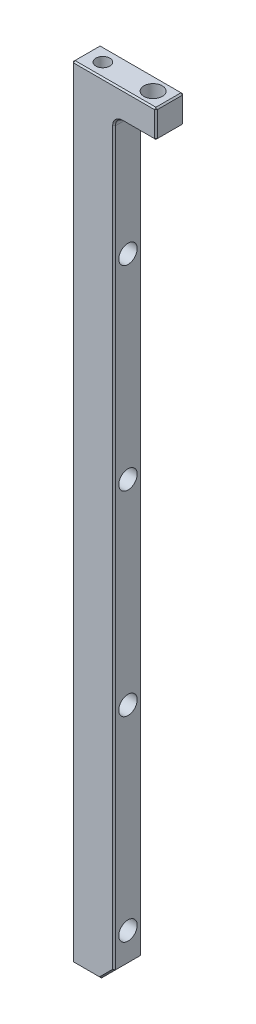
from build123d import *

# Parameters (mm, degrees)
SKETCH_1_W          = 30
SKETCH_1_H          = 280
EXTRUDE_1_DEPTH     = 5
SKETCH_2_W          = 15
SKETCH_2_H          = 270
CUT_EXTRUDE_1_DEPTH = 142.155942135
FILLET_1_R          = 3
HOLE_WIZARD_M6_1_D  = 6.6
CHAMFER_1_SIZE      = 5
HOLE_WIZARD_M6_2_D  = 6.6
CHAMFER_2_SIZE      = 0.5
F_5_0MM_1_D         = 5
F_5_0MM_1_DEPTH     = 6
F_5_0MM_1_TIP       = 1.502151548


with BuildPart() as part:
    # 草图1 → 凸台-拉伸1 (new, symmetric)
    with BuildSketch(Plane.XY):
        Rectangle(SKETCH_1_W, SKETCH_1_H)
    extrude(amount=EXTRUDE_1_DEPTH, both=True)

    # 草图2 → 切除-拉伸1 (cut, through all)
    with BuildSketch(Plane(origin=(0, 0, -5), x_dir=(-1, 0, 0), z_dir=(0, 0, -1))):
        with Locations((-7.5, -5)):
            Rectangle(SKETCH_2_W, SKETCH_2_H)
    extrude(amount=-CUT_EXTRUDE_1_DEPTH, mode=Mode.SUBTRACT)

    # 圆角1
    fillet_1_edges = [part.edges().sort_by_distance(p)[0] for p in [
        (0, 130, 0),
    ]]
    fillet(fillet_1_edges, radius=FILLET_1_R)

    # M6 间隙孔1 (through all)
    with Locations(Plane(origin=(0, 130, 0), x_dir=(-1, 0, 0), z_dir=(0, -1, 0))):
        with Locations((-9, 0)):
            Hole(HOLE_WIZARD_M6_1_D / 2)

    # 倒角1
    chamfer_1_edges = [part.edges().sort_by_distance(p)[0] for p in [
        (0, -140, 0),
    ]]
    chamfer(chamfer_1_edges, length=CHAMFER_1_SIZE)

    # M6 间隙孔2 (through all)
    with Locations(Plane(origin=(0, 0, 0), x_dir=(0, 0, -1), z_dir=(1, 0, 0))):
        with Locations((0, 85), (0, 15), (0, -55), (0, -125)):
            Hole(HOLE_WIZARD_M6_2_D / 2)

    # 倒角2
    chamfer_2_edges = [part.edges().sort_by_distance(p)[0] for p in [
        (-15, 0, 5),
        (-10, -140, 5),
        (15, 135, -5),
        (15, 135, 5),
        (15, 130, 0),
        (9, 130, -5),
        (9, 130, 5),
        (0.878679656, 129.121320344, -5),
        (0.878679656, 129.121320344, 5),
        (0, -4, -5),
        (0, -4, 5),
        (-2.5, -137.5, -5),
        (-10, -140, -5),
        (-2.5, -137.5, 5),
        (-15, 0, -5),
        (0, 140, -5),
        (0, 140, 5),
        (-15, -140, 0),
        (-15, 140, 0),
        (15, 140, 0),
    ]]
    chamfer(chamfer_2_edges, length=CHAMFER_2_SIZE)

    # Ø5.0mm 暗销孔1
    with Locations(Plane(origin=(0, 140, 0), x_dir=(1, 0, 0), z_dir=(0, 1, 0))):
        with Locations((-9, 0)):
            Hole(F_5_0MM_1_D / 2, depth=F_5_0MM_1_DEPTH)
            with Locations((0, 0, -(F_5_0MM_1_DEPTH + F_5_0MM_1_TIP / 2))):  # 118° drill point
                Cone(0, F_5_0MM_1_D / 2, F_5_0MM_1_TIP, mode=Mode.SUBTRACT)


solid = part.part
